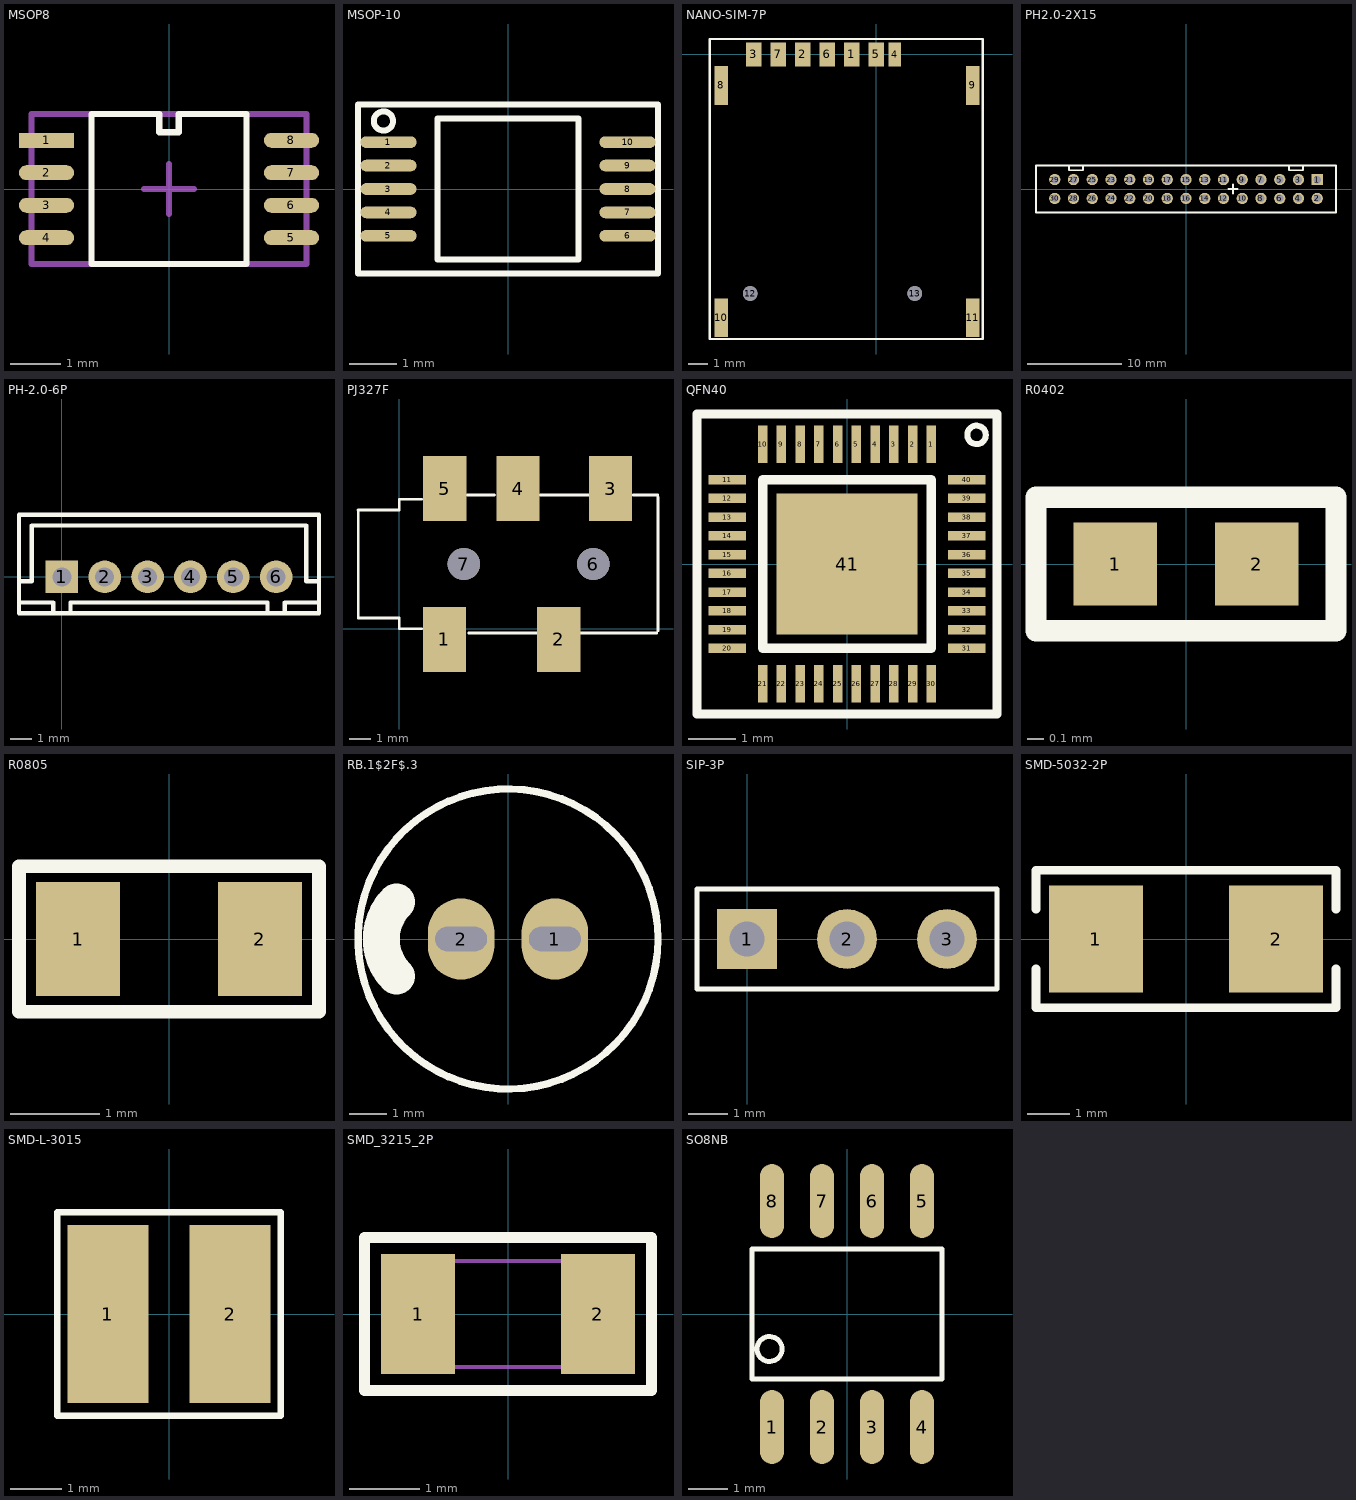
[diagram p0: the footprints below, top view; thin cyan lines are the x and y axes]
# Altium footprint library MISC82162-2.PcbLib: 66 footprints (part 3 of 5)
Each footprint in its own frame and in the unit in brackets; x right, y up, seen from the top. Pads: shape width x height; smd on the part's side, far side on the other; paste and mask are expansions set on the pad; w line width, h text height; cw(c..) or ccw(c..) is an arc to the next point about the centre after c.

## MSOP8 [mm]
pads (8):
  rect 1.1x0.3 smd: 1(-2.45,0.975)
  oval 1.1x0.3 smd: 2(-2.45,0.325) 3(-2.45,-0.325) 4(-2.45,-0.975) 5(2.45,-0.975) 6(2.45,-0.325) 7(2.45,0.325) 8(2.45,0.975)
Top Overlay:
  lines w0.127: -1.55,-1.5 -1.55,1.5 -0.194,1.5 -0.194,1.138 0.194,1.138 0.194,1.5 1.55,1.5 1.55,-1.5 -1.55,-1.5
Mechanical 20:
  lines w0.127: -0.5,0 0,0 ; 0,-0.5 0,0 ; 0,0.5 0,0 ; 0.5,0 0,0 ; -2.75,-1.5 -2.75,1.5 2.75,1.5 2.75,-1.5 -2.75,-1.5

## MSOP-10 [mm]
height 1.27
pads (10):
  oval 1.2x0.25 smd paste-0.1 mask-0.1: 1(-2.55,1) 2(-2.55,0.5) 3(-2.55,0) 4(-2.55,-0.5) 5(-2.55,-1) 6(2.55,-1) 7(2.55,-0.5) 8(2.55,0) 9(2.55,0.5) 10(2.55,1)
Top Overlay:
  circle w0.127: c-2.658,1.45 r0.204
  lines w0.127: -3.2,-1.8 3.2,-1.8 3.2,1.8 -3.2,1.8 -3.2,-1.8 ; -1.5,-1.5 1.5,-1.5 1.5,1.5 -1.5,1.5 -1.5,-1.5

## NANO-SIM-7P [mm]
pads (13):
  rect 0.8x1.23 smd: 1(-1.27,0) 2(-3.81,0) 3(-6.35,0) 5(0,0) 6(-2.54,0) 7(-5.08,0)
  rect 0.65x1.23 smd: 4(0.95,0)
  rect 0.7x2 smd: 8(-8.02,-1.6) 9(4.98,-1.6) 10(-8.02,-13.6) 11(4.98,-13.6)
  round 0.75 hole 0.75 unplated: 12(-6.52,-12.349) 13(1.98,-12.349)
Top Overlay:
  lines w0.127: -8.6,-14.7 -8.6,0.8 5.5,0.8 5.5,-14.7 -8.6,-14.7

## PCBComponent_1 [mm]

## PH2.0-2X15 [mm]
pads (30):
  rect 1.2x1.2 / inner round 1.2 / far side rect 1.2x1.2 hole 0.8: 1(14,1)
  round 1.2 hole 0.8: 2(14,-1) 3(12,1) 4(12,-1) 5(10,1) 6(10,-1) 7(8,1) 8(8,-1) 9(6,1) 10(6,-1) 11(4,1) 12(4,-1) 13(2,1) 14(2,-1) 15(0,1) 16(0,-1) 17(-2,1) 18(-2,-1) 19(-4,1) 20(-4,-1) 21(-6,1) 22(-6,-1) 23(-8,1) 24(-8,-1) 25(-10,1) 26(-10,-1) 27(-12,1) 28(-12,-1) 29(-14,1) 30(-14,-1)
Top Overlay:
  lines w0.2: 4.5,0 5,0 ; 5,-0.5 5,0 ; 5,0.5 5,0 ; 5.5,0 5,0 ; -16,-2.5 -16,2.5 16,2.5 16,-2.5 -16,-2.5
  lines w0.203: -12.5,2 -12.5,2.5 -11,2.5 -11,2 -12.5,2 ; 11,2 11,2.5 12.5,2.5 12.5,2 11,2

## PH-2.0-6P [mil]
pads (6):
  rect 60x60 / inner round 60 / far side rect 60x60 hole 35: 1(0,0)
  round 60 hole 35: 2(78.74,0) 3(157.48,0) 4(236.22,0) 5(314.96,0) 6(393.7,0)
Top Overlay:
  lines w8: -78.74,-47.24 -15.75,-47.24 -15.75,-62.99 ; -78.74,-7.87 -55.12,-7.87 -55.12,94.49 448.82,94.49 448.82,-7.87 472.44,-7.87 ; 15.75,-62.99 15.75,-47.24 377.95,-47.24 377.95,-62.99 ; 409.45,-66.93 409.45,-47.24 472.44,-47.24 ; -78.74,-66.93 -78.74,114.17 472.44,114.17 472.44,-66.93 -78.74,-66.93
Bottom Overlay:
  region: 47.24,-39.37 31.5,-39.37 31.5,39.37 47.24,39.37
  region: 125.98,-39.37 110.24,-39.37 110.24,39.37 125.98,39.37
  region: 204.72,-39.37 188.98,-39.37 188.98,39.37 204.72,39.37
  region: 283.46,-39.37 267.72,-39.37 267.72,39.37 283.46,39.37
  region: 362.2,-39.37 346.46,-39.37 346.46,39.37 362.2,39.37

## PJ327F [mm]
pads (7):
  rect 2x3 smd paste+0.3: 1(2.1,-0.5) 2(7.4,-0.5) 3(9.8,6.5) 4(5.51,6.5) 5(2.11,6.5)
  round 1.5 hole 1.5 unplated: 6(9,3) 7(3,3)
Top Overlay:
  lines w0.127: -1.91,5.5 0,5.5 0,6 1.05,6 ; -1.9,5.5 -1.9,0.5 0,0.5 0,0 1.05,0 ; 3.16,6.2 3.69,6.2 3.69,6.198 4.42,6.198 ; 3.22,-0.2 6.35,-0.2 ; 6.528,6.198 8.763,6.198 ; 8.407,-0.2 11.941,-0.2 ; 10.846,6.198 11.989,6.198 ; 12,-0.1 12,6.1

## QFN40 [mm]
pads (41):
  rect 0.2x0.8 smd paste+0.05: 1(1.8,2.55) 2(1.4,2.55) 3(1,2.55) 4(0.6,2.55) 5(0.2,2.55) 6(-0.2,2.55) 7(-0.6,2.55) 8(-1,2.55) 9(-1.4,2.55) 10(-1.8,2.55) 21(-1.8,-2.55) 22(-1.4,-2.55) 23(-1,-2.55) 24(-0.6,-2.55) 25(-0.2,-2.55) 26(0.2,-2.55) 27(0.6,-2.55) 28(1,-2.55) 29(1.4,-2.55) 30(1.8,-2.55)
  rect 0.8x0.2 smd paste+0.05: 11(-2.55,1.8) 12(-2.55,1.4) 13(-2.55,1) 14(-2.55,0.6) 15(-2.55,0.2) 16(-2.55,-0.2) 17(-2.55,-0.6) 18(-2.55,-1) 19(-2.55,-1.4) 20(-2.55,-1.8) 31(2.55,-1.8) 32(2.55,-1.4) 33(2.55,-1) 34(2.55,-0.6) 35(2.55,-0.2) 36(2.55,0.2) 37(2.55,0.6) 38(2.55,1) 39(2.55,1.4) 40(2.55,1.8)
  rrect0% 3x3 smd: 41(0,0)
Top Overlay:
  circle w0.127: c2.764,2.754 r0.198
  lines w0.2: -3.2,-3.2 3.2,-3.2 3.2,3.2 -3.2,3.2 -3.2,-3.2 ; -1.8,-1.8 1.8,-1.8 1.8,1.8 -1.8,1.8 -1.8,-1.8

## R0402 [mm]
height 0.432
pads (2):
  rect 0.5x0.5 smd mask+0.05: 1(-0.425,0) 2(0.425,0)
Top Overlay:
  lines w0.127: -0.9,-0.4 -0.9,0.4 0.9,0.4 0.9,-0.4 -0.9,-0.4

## R0805 [mil]
pads (2):
  rect 37x50 smd: 1(-40,0) 2(40,0)
Top Overlay:
  lines w6: -66,-32 66,-32 66,32 -66,32 -66,-32

## RB.1$2F$.3 [mm]
pads (2):
  oval 1.8x2.2 hole 0.66 slot 1.4 at 0 deg: 1(1.27,0) 2(-1.27,0)
Top Overlay:
  circle w0.2: c0,0 r4.064
  lines w1: -3.02,-1.009 cw(c-2.015,-0.004) -3.02,1.001
Bottom Overlay:
  region: -0.2,1.7 0.2,1.7 0.2,-1.5 -0.2,-1.5

## SIP-3P [mil]
pads (3):
  rect 60x60 / inner round 60 / far side rect 60x60 hole 35: 1(0,0)
  round 60 hole 35: 2(100,0) 3(200,0)
Top Overlay:
  lines w5: -50,-50 250,-50 250,50 -50,50 -50,-50

## SMD-5032-2P [mm]
pads (2):
  rect 2.2x2.5 smd: 1(-2.1,0) 2(2.1,0)
Top Overlay:
  lines w0.2: -3.5,-0.7 -3.5,-1.6 3.5,-1.6 3.5,-0.7 ; -3.5,0.7 -3.5,1.6 3.5,1.6 3.5,0.7

## SMD-L-3015 [mm]
pads (2):
  rect 1.6x3.5 smd: 1(-1.2,0) 2(1.2,0)
Top Overlay:
  lines w0.127: -2.2,-2 2.2,-2 2.2,2 -2.2,2 -2.2,-2

## SMD_3215_2P [mm]
pads (2):
  rect 1.049x1.699 smd mask+0.051: 1(-1.27,0) 2(1.27,0)
Top Overlay:
  lines w0.152: -2.029,-1.079 -2.029,1.079 2.029,1.079 2.029,-1.079 -2.029,-1.079
Mechanical 20:
  lines w0.051: -1.6,-0.749 -1.6,0.749 1.6,0.749 1.6,-0.749 -1.6,-0.749

## SO8NB [mil]
pads (8):
  oval 24x74 smd: 1(-75,-113) 2(-25,-113) 3(25,-113) 4(75,-113) 5(75,113) 6(25,113) 7(-25,113) 8(-75,113)
Top Overlay:
  circle w5: c-77.5,-35 r12.5
  lines w5: -95,-65 95,-65 95,65 -95,65 -95,-65